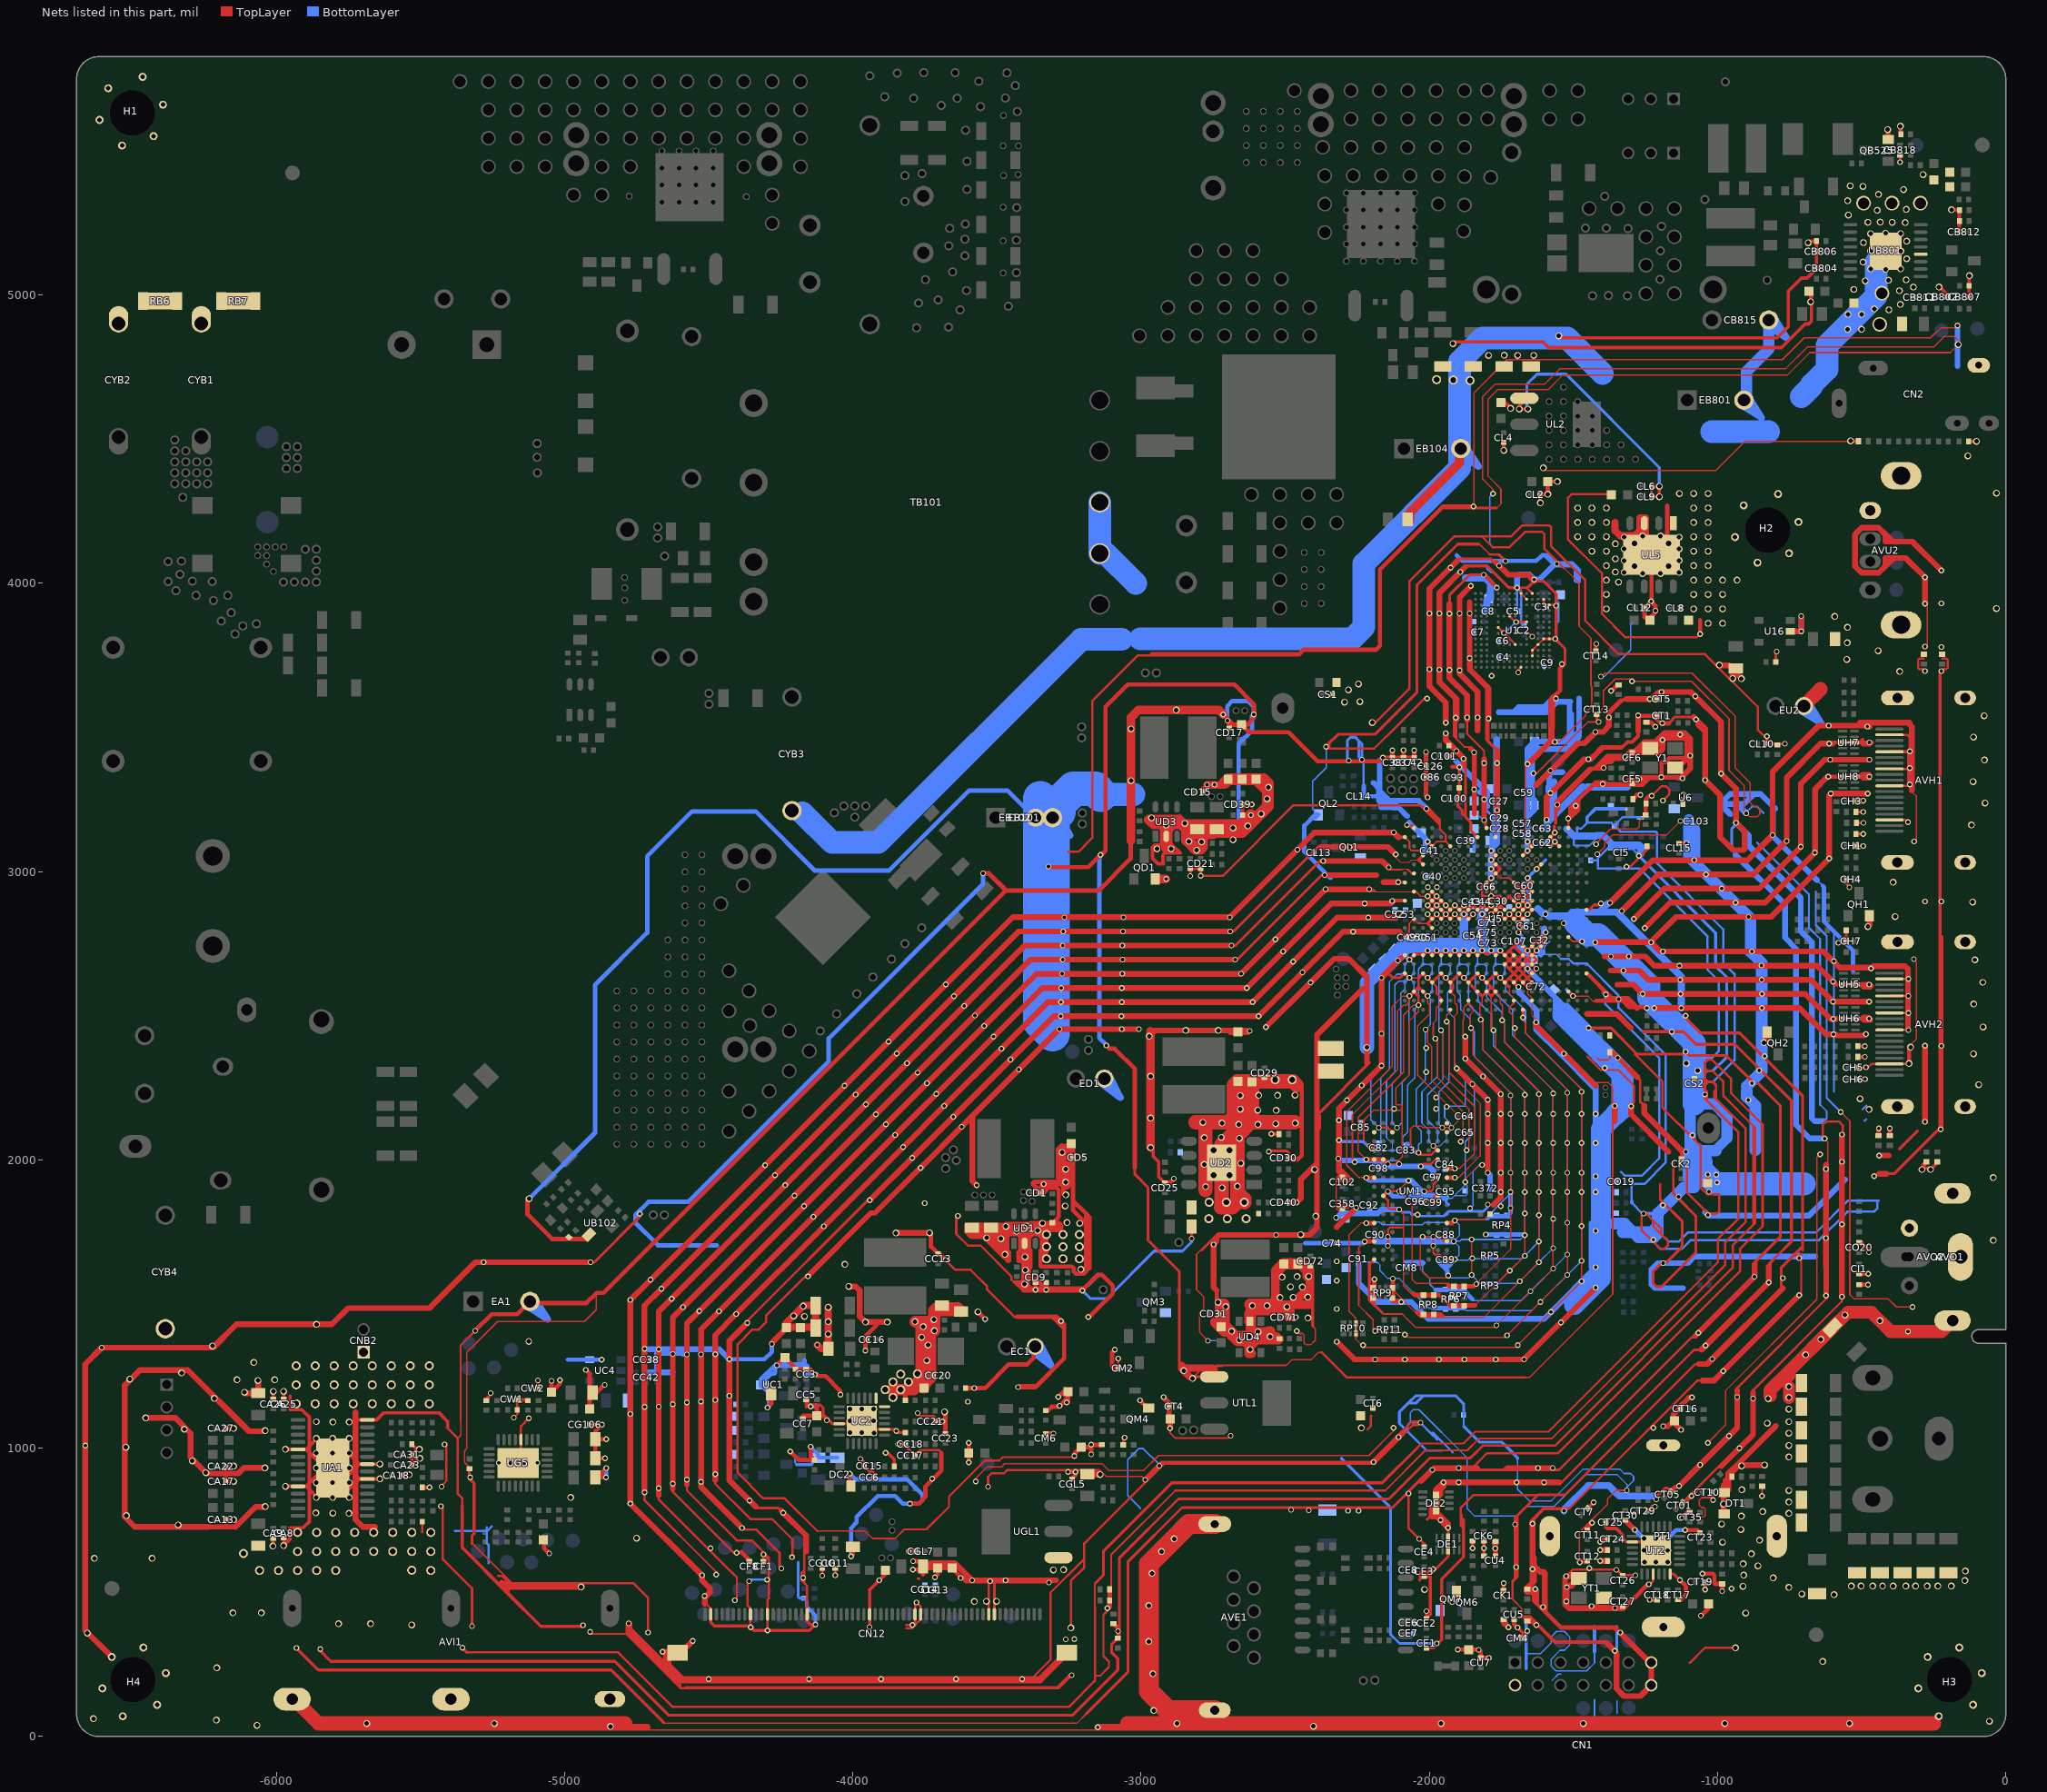
[diagram p0: the nets of this part, all layers, seen from the top]
# Altium PCB MISC84395.PcbDoc (part 13 of 26)
Units mil, origin at the board's own origin, x right, y up, seen from the top; angles counter-clockwise.
Board outline 6692.91 x 5826.77 mil, 2 copper layers (TopLayer, BottomLayer), stack 61.855 mil thick; 951 components, 565 nets, 4374 pads, 1804 vias.
Unrouted connection lines stored in the file: 1.

## Via types
v1: diameter 19.68, hole 11.81, TopLayer to BottomLayer, tented both sides, 1262 vias
v2: diameter 23.62, hole 15.75, TopLayer to BottomLayer, tented both sides, 524 vias
v3: diameter 31.5, hole 19.68, TopLayer to BottomLayer, tented both sides, 11 vias
v4: diameter 24, hole 16, TopLayer to BottomLayer, tented both sides, 6 vias
v5: diameter 19, hole 11.81, TopLayer to BottomLayer, tented both sides, 1 vias

## Nets (pads, with @x,y where several pads share a name; then routed paths per layer and width w, separated by ;. In a path a pad name is that pad's centre, name@x,y a point inside that pad or via, vN(x,y) a via of type N, cw(c..) or ccw(c..) an arc to the next point about the centre after c; other vN are vias at no path point) (continued)
GND: AVE1.9 AVE1.10 AVH1.2 AVH1.5 AVH1.8 AVH1.11 AVH1.17 AVH1.20 AVH1.21 AVH1.22 AVH1.23 AVH2.2 AVH2.5 AVH2.8 AVH2.11 AVH2.17 AVH2.20 AVH2.21 AVH2.22 AVH2.23 AVI1.2 AVI1.4 AVI1.6 AVO1.2 AVO2.3 AVO2.4 AVO2.5 AVU2.4 AVU2.5 AVU2.6 C1.1 C2.1 C3.1 C4.1 C5.1 C6.1 C7.1 C8.1 C9.2 C25.1 C26.1 C27.1 C28.1 C29.1 C30.1 C31.1 C32.1 C33.1 C34.1 C35.1 C36.1 C37.1 C38.1 C39.1 C40.1 C41.1 C42.1 C43.1 C44.1 C45.1 C46.1 C47.1 C48.1 C49.1 C50.1 C51.1 C52.1 C53.1 C54.2 C55.1 C56.1 C57.1 C58.1 C59.1 C60.1 C61.1 C62.1 C63.1 C64.2 C65.1 C66.2 C71.1 C72.1 C73.1 C74.1 C75.1 C80.1 C81.1 C82.1 C83.1 C84.1 C85.1 C86.2 C87.1 C88.1 C89.1 C90.1 C91.1 C92.1 C93.1 C94.1 C95.1 C96.1 C97.1 C98.1 C99.1 C100.1 C101.2 C102.2 C103.1 C104.1 C105.1 C106.1 C107.1 C108.1 C126.2 C358.1 C372.1 CA1.1 CA2.1 CA8.1 CA9.1 CA13.1 CA17.2 CA18.2 CA22.1 CA23.2 CA25.2 CA26.1 CA27.2 CA31.2 CB802.1 CB803.1 CB804.1 CB805.1 CB806.1 CB807.2 CB811.2 CB812.1 CB813.1 CB814.2 CB815.2 CB816.2 CB818.1 CB819.2 CC1.1 CC2.1 CC3.2 CC4.2 CC5.2 CC6.1 CC7.1 CC8.2 CC9.2 CC10.2 CC11.2 CC12.2 CC13.1 CC14.1 CC15.1 CC16.1 CC17.1 CC18.1 CC19.2 CC20.1 CC21.2 CC22.2 CC23.1 CC28.2 CC29.2 CC30.2 CC33.1 CC34.1 CC36.2 CC38.2 CC42.2 CC43.1 CD1.1 CD2.1 CD4.2 CD5.2 CD6.2 CD8.1 CD9.2 CD13.2 CD14.2 CD15.2 CD17.2 CD18.2 CD19.2 CD20.2 CD21.2 CD23.1 CD24.1 CD25.1 CD26.1 CD28.1 CD29.2 CD30.2 CD31.1 CD39.2 CD40.2 CD45.2 CD69.1 CD71.1 CD72.1 CD73.2 CD74.2 CE1.1 CE2.1 CE3.1 CE4.1 CE5.2 CE6.1 CE7.1 CE8.2 CF1.1 CF5.2 CF6.2 CF8.1 CG1.2 CG2.2 CG3.2 CG10.1 CG11.1 CG12.1 CG13.1 CG14.1 CG103.1 CG104.2 CG105.1 CG106.1 CGL4.1 CGL5.2 CGL6.2 CGL7.2 CGL49.2 CH1.2 CH3.1 CH4.1 CH5.2 CH6.1 CH7.1 CI1.1 CI5.1 CK1.2 CK2.2 CK6.1 CL1.1 CL2.2 CL3.2 CL4.2 CL5.1 CL6.1 CL7.1 CL8.1 CL9.1 CL10.1 CL11.2 CL12.2 CL13.1 CL14.1 CL15.1 CM2.2 CM3.1 CM4.1 CM6.1 CM7.1 CM8.1 CM9.1 CN1.2 CN1.13 CN1.14 CN2.1 CN12.2 CN12.9 CN12.12 CN12.19 CN12.30 CN12.38 CN12.39 CN12.51 CN12.52 CN12.61 CN12.62 CNB2.1 CO19.1 CO20.1 CS1.2 CS2.2 CT01.1 CT1.2 CT3.1 CT4.2 CT05.1 CT5.1 CT6.1 CT7.1 CT8.2 CT10.1 CT11.1 CT12.1 CT13.1 CT14.2 CT15.1 CT16.1 CT17.1 CT18.2 CT19.2 CT23.2 CT24.2 CT25.1 CT26.1 CT27.1 CT29.1 CT30.1 CT35.2 CT41.1 CT42.1 CT43.1 CT44.1 CT45.1 CT46.1 CT47.1 CT48.1 CT49.1 CT50.1 CT55.1 CT67.1 CT68.1 CT70.1 CU1.1 CU4.1 CU5.1 CU6.2 CU7.2 CU.2 CW1.1 CW2.2 CYB1.2 CYB2.2 CYB3.2 CYB4.2 D4.A D5.A D11.A D12.A D13.A D14.A DA1.A DA2.A DC2.3 DE1.GND DE2.EPAD@-1977,809.63 DH1.A DH2.A DH3.A DH4.A DH5.A DH6.A DI1.A DI2.A DI04.A DI4.A DK1.A DK3.A DO1.A DO7.A DT1.1 DT1.3 DT2.A DT3.A DT4.A DU1.A DU2.A DU3.A DU4.A DU5.A DU6.A DU7.A DU8.A DU9.A DV1.A DV2.A DV3.A DV4.A EA1.2 EB101.2 EB102.2 EB104.2 EB801.2 EC1.2 ED1.2 EU2.2 GND_JP1.JP_2K GND_JP2.JP_2K H1.1 H1.2 H1.3 H1.4 H1.5 H1.6 H2.1 H2.2 H2.3 H2.4 H2.5 H2.6 H3.1 H3.2 H3.3 H3.4 H3.5 H3.6 H4.1 H4.2 H4.3 H4.4 H4.5 H4.6 L3.2 LT2.2 LT5.1 MR313.1 P1.1 P1.2 pad.VIA5@-296.76,5318.37 pad.VIA5@-321,5027 pad.VIA5@-344.19,5125.37 pad.VIA5@-344.19,5186.37 pad.VIA5@-345.69,5296.87 pad.VIA5@-346.19,5052.37 pad.VIA5@-349.69,5250.87 pad.VIA5@-355,5365 pad.VIA5@-366.19,4967.37 pad.VIA5@-369.19,5014.37 pad.VIA5@-394.69,5251.79 pad.VIA5@-395.19,5318.37 pad.VIA5@-406,4948 pad.VIA5@-407.19,5050.87 pad.VIA5@-430.19,5005.87 pad.VIA5@-436.19,5252.37 pad.VIA5@-438,4898 pad.VIA5@-442,5349 pad.VIA5@-446.19,5293.37 pad.VIA5@-457,4952 pad.VIA5@-479.19,5251.87 pad.VIA5@-488.19,5048.37 pad.VIA5@-493.61,5318.37 pad.VIA5@-494.19,5181.37 pad.VIA5@-495.19,5113.87 pad.VIA5@-496,5376 pad.VIA5@-501,4881 pad.VIA5@-501,4933 pad.VIA5@-528,5019 pad.VIA5@-540,5378 pad.VIA5@-546.69,5276.87 pad.VIA5@-548,4933 pad.VIA5@-549,4881 pad.VIA5@-549.19,5326.87 pad.VIA5@-933.04,4011 pad.VIA5@-983.04,3861 pad.VIA5@-983.04,3911 pad.VIA5@-983.04,3961 pad.VIA5@-983.04,4011 pad.VIA5@-1033.04,3861 pad.VIA5@-1033.04,3911 pad.VIA5@-1033.04,3961 pad.VIA5@-1033.04,4011 pad.VIA5@-1033.04,4061 pad.VIA5@-1033.04,4111 pad.VIA5@-1033.04,4161 pad.VIA5@-1033.04,4211 pad.VIA5@-1033.04,4261 pad.VIA5@-1033.04,4311 pad.VIA5@-1083.04,3911 pad.VIA5@-1083.04,3961 pad.VIA5@-1083.04,4011 pad.VIA5@-1083.04,4061 pad.VIA5@-1083.04,4111 pad.VIA5@-1083.04,4161 pad.VIA5@-1083.04,4211 pad.VIA5@-1083.04,4261 pad.VIA5@-1083.04,4311 pad.VIA5@-1133.04,4311 pad.VIA5@-1344,4004 pad.VIA5@-1355,4039 pad.VIA5@-1355,4084.5 pad.VIA5@-1355,4137 pad.VIA5@-1386,3911 pad.VIA5@-1386,3961 pad.VIA5@-1386,4011 pad.VIA5@-1386,4061 pad.VIA5@-1386,4111 pad.VIA5@-1386,4161 pad.VIA5@-1386,4211 pad.VIA5@-1386,4261 pad.VIA5@-1436,4111 pad.VIA5@-1436,4161 pad.VIA5@-1436,4211 pad.VIA5@-1436,4261 pad.VIA5@-1486,4161 pad.VIA5@-1486,4211 pad.VIA5@-1486,4261 pad.VIA5@-1638,4790 pad.VIA5@-1694,4790 pad.VIA5@-1740,4791 pad.VIA5@-1795,4790 pad.VIA5@-1859,4703 pad.VIA5@-1917,4705 pad.VIA5@-1975,4706 pad.VIA5@-2476,2278 pad.VIA5@-2535,2278 pad.VIA5@-2636,1796 pad.VIA5@-2642,1853 pad.VIA5@-2681,3110 pad.VIA5@-2701,1796 pad.VIA5@-2704,1853 pad.VIA5@-2764,1853 pad.VIA5@-2765,1796 pad.VIA5@-2790,3103 pad.VIA5@-2807,3074 pad.VIA5@-2834,3105 pad.VIA5@-2848,3166.69 pad.VIA5@-2895.85,3078.43 pad.VIA5@-2913,3161 pad.VIA5@-2944.83,3078.43 pad.VIA5@-2964,3186 pad.VIA5@-3214,1657 pad.VIA5@-3214,1699 pad.VIA5@-3214,1741 pad.VIA5@-3271,1657 pad.VIA5@-3271,1699 pad.VIA5@-3271,1741 pad.VIA5@-3328,1657 pad.VIA5@-3328,1699 pad.VIA5@-3328,1741 pad.VIA5@-3776,1258 pad.VIA5@-3807,1230 pad.VIA5@-3833.87,1203.13 pad.VIA5@-3833.87,1256.87 pad.VIA5@-3860.74,1176.26 pad.VIA5@-3860.74,1230 pad.VIA5@-3887.61,1203.13 pad.VIA5@-5463.94,576 pad.VIA5@-5463.94,642 pad.VIA5@-5463.94,708 pad.VIA5@-5468.95,1154 pad.VIA5@-5468.95,1220 pad.VIA5@-5468.95,1286 pad.VIA5@-5529.94,642 pad.VIA5@-5529.94,708 pad.VIA5@-5530,577 pad.VIA5@-5534.95,1154 pad.VIA5@-5534.95,1220 pad.VIA5@-5534.95,1286 pad.VIA5@-5595.94,642 pad.VIA5@-5595.94,708 pad.VIA5@-5600.95,1154 pad.VIA5@-5600.95,1220 pad.VIA5@-5600.95,1286 pad.VIA5@-5661.94,642 pad.VIA5@-5661.94,708 pad.VIA5@-5666.94,1154 pad.VIA5@-5666.94,1220 pad.VIA5@-5666.95,1286 pad.VIA5@-5727.94,642 pad.VIA5@-5727.94,708 pad.VIA5@-5732.94,1154 pad.VIA5@-5732.94,1220 pad.VIA5@-5732.94,1286 pad.VIA5@-5793.94,576 pad.VIA5@-5793.94,642 pad.VIA5@-5793.94,708 pad.VIA5@-5798.94,1154 pad.VIA5@-5798.94,1220 pad.VIA5@-5798.94,1286 pad.VIA5@-5859.94,576 pad.VIA5@-5859.94,642 pad.VIA5@-5859.94,708 pad.VIA5@-5864.94,1154 pad.VIA5@-5864.94,1220 pad.VIA5@-5864.94,1286 pad.VIA5@-5925.94,576 pad.VIA5@-5925.94,642 pad.VIA5@-5925.94,708 pad.VIA5@-5930.94,1154 pad.VIA5@-5930.94,1220 pad.VIA5@-5930.94,1286 pad.VIA5@-5991.94,576 pad.VIA5@-6057.94,576 pad.VIA5@-6113.94,635 PT1.1 PT1.2 PT1.3 PT1.4 QB525.E QD1.S QH1.E QH2.E QL1.E QL2.E QM3.E QM4.E QM6.E QM7.E R3.1 R11.1 R26.1 R28.1 R33.1 R37.1 R47.1 R49.2 R50.2 R52.1 RA19.1 RA21.1 RA31.1 RB6.1 RB6.2 RB6.3 RB7.1 RB7.2 RB7.3 RB134.1 RB140.2 RB803.1 RB812.1 RB818.2 RB819.2 RB820.2 RB821.2 RB822.1 RB827.1 RB834.1 RC3.1 RC7.2 RC12.1 RC17.1 RC18.1 RC24.1 RC26.1 RC27.1 RC31.1 RD4.1 RD9.1 RD16.1 RD27.2 RD28.2 RD51.1 RG2.1 RG3.1 RG4.1 RG7.2 RG8.2 RG9.2 RG30.2 RI5.1 RI9.2 RI12.2 RL8.1 RL10.2 RL11.2 RM3.2 RM9.2 RM11.1 RM14.2 RO4.1 RP3.5 RP3.6 RP4.1 RP4.2 RP4.7 RP4.8 RP5.3 RP5.4 RP6.1 RP6.2 RP6.7 RP6.8 RP7.1 RP7.2 RP7.7 RP7.8 RP8.1 RP8.2 RP8.7 RP8.8 RP9.1 RP9.2 RP9.7 RP9.8 RP10.3 RP10.4 RP11.5 RP11.6 RS1.1 RS2.2 RU10.1 RW2.1 TB101.8 TB101.9 U1.A6 U1.C4 U1.D4 U1.E3 U1.E7 U1.F1 U1.F2 U1.G5 U1.H10 U1.J5 U1.K8 U1.M1 U1.M2 U1.N2 U1.N5 U1.P4 U1.P6 U5.A8 U5.A16 U5.AA3 U5.AA12 U5.AA20 U5.B7 U5.B9 U5.B14 U5.B17 U5.C3 U5.C11 U5.C12 U5.C13 U5.C16 U5.C19 U5.C20 U5.D7 U5.D8 U5.D9 U5.D10 U5.D12 U5.D14 U5.D16 U5.D18 U5.E1 U5.E7 U5.E11 U5.E13 U5.E15 U5.E17 U5.E19 U5.E21 U5.F7 U5.F8 U5.F9 U5.F10 U5.G7 U5.G8 U5.G9 U5.G10 U5.G11 U5.G13 U5.G14 U5.G15 U5.G16 U5.G17 U5.G18 U5.G19 U5.G20 U5.G21 U5.H6 U5.H7 U5.H8 U5.J3 U5.J6 U5.J21 U5.K8 U5.K18 U5.L8 U5.L9 U5.L10 U5.L12 U5.L14 U5.L15 U5.L16 U5.L17 U5.L18 U5.L20 U5.M1 U5.M7 U5.M8 U5.M9 U5.M10 U5.M11 U5.M12 U5.M13 U5.M14 U5.M15 U5.M16 U5.M17 U5.M18 U5.N7 U5.N8 U5.N9 U5.N10 U5.N17 U5.N18 U5.N21 U5.P7 U5.P8 U5.P18 U5.P20 U5.R7 U5.R9 U5.R12 U5.R21 U5.T11 U5.T20 U5.U6 U5.U11 U5.U19 U5.V8 U5.V11 U5.V19 U5.W4 U5.W5 U5.W7 U5.W16 U5.W18 U5.Y5 U5.Y11 U5.Y13 U5.Y21 U6.1 U16.2 UA1.6 UA1.8 UA1.14 UA1.19 UA1.24 UA1.EPAD UB102.A UB801.4 UB801.17 UC1.3 UC2.4 UC2.14 UC2.18 UC2.19 UC2.25 UC4.5 UD1.2 UD2.9 UD3.2 UD4.2 UG5.4 UG5.EPAD UGL1.1 UH5.GND UH6.GND UH7.GND UH8.GND UL2.1 UL5.1 UL5.3 UL5.EPAD UM1.A9 UM1.B1 UM1.B3 UM1.B9 UM1.D1 UM1.D8 UM1.E1 UM1.E2 UM1.E8 UM1.F9 UM1.G1 UM1.G8 UM1.G9 UM1.J2 UM1.J8 UM1.M1 UM1.M9 UM1.P1 UM1.P9 UM1.T1 UM1.T9 UT2.14 UT2.21 UT2.24 UT2.25 UTL1.1 Y1.2 Y1.4 YT1.2 YT1.4 | length 337716.2
  TopLayer w3.94: v1@-2216.58,2939.92 -2215.26,2938.6 -2207.22,2930.57 -2195.87,2930.57 ; v1@-2206.34,2941.05 -2195.87,2930.57 ; -2137.21,2886.78 -2134.38,2889.6 v1@-2129.06,2894.93 ; v1@-2122.15,3054.24 -2100.84,3032.93 -2069.18,3032.93 -2061.31,3040.81 -2037.68,3040.81 ; -2097.22,3006.58 -2094.49,3009.31 -2077.05,3009.31 -2075.46,3007.72 -2061.31,2993.56 U5.T20@-2053.43,2993.56 ; -2081.98,2536.87 -2080.99,2536.87 -2069.18,2548.68 v1(-2069.18,2568.36) ; -2070.66,2522.6 -2070.66,2523.58 -2057.37,2536.87 v1(-2037.69,2536.87) ; U5.P20@-2053.43,2930.57 -2184.51,2930.57 ; U5.V19@-2023.9,3056.56 U5.V19@-2021.94,3056.56 ; v1(-2006.19,2568.36) -2006.19,2544.74 -2000.28,2538.84 -2000.28,2504.88 -2000.78,2504.39 ; -1977.16,2483.72 -1976.66,2484.21 -1976.66,2527.02 -1958.95,2544.74 U5.B17@-1958.94,2552.62 ; U5.C16@-1927.45,2584.12 -1911.7,2568.36 -1911.7,2544.74 -1903.83,2536.87 -1903.83,2507.83 -1904.32,2507.34 ; -1880.7,2486.67 -1880.21,2487.16 -1880.21,2528.99 -1864.46,2544.74 ; U5.B14@-1864.46,2552.62 -1864.46,2544.74 ; -1849.2,2513.25 -1848.71,2513.74 -1848.71,2528.99 -1864.46,2544.74 ; -1824.6,2506.85 -1825.09,2507.34 -1825.09,2536.87 -1817.21,2544.74 -1817.21,2568.36 ; U5.Y11@-1769.97,3119.55 -1769.97,3196.08 ; v1(-1747.82,2484.21) -1746.35,2485.69 -1746.35,2536.87 -1754.22,2544.74 -1754.22,2568.36 ; -1722.23,2512.75 -1722.73,2513.25 -1722.73,2528.99 -1706.98,2544.74 U5.B9@-1706.98,2552.62 ; -1667.47,3182.22 -1667.61,3182.08 -1667.61,3135.3 -1659.73,3127.42 v1(-1659.73,3103.8) ; U5.B7@-1643.98,2552.62 -1643.98,2500.95 -1641.52,2498.49 ; -2195.87,2930.57 -2189.65,2930.57 ; -2195.87,2930.57 -2195.87,2936.79 ; -2195.87,2936.79 -2189.65,2930.57 ; -2195.87,2936.79 -2195.87,2937.74 ; -2195.87,2937.74 -2195.65,2937.74 -2188.48,2930.57 ; -2195.87,2937.74 -2195.87,2941.93 -2184.51,2930.57 ; -2189.65,2930.57 -2188.48,2930.57 ; -2188.48,2930.57 -2184.51,2930.57 ; -1754.22,2568.36 U5.C11@-1769.97,2584.12 -1754.22,2568.36
  TopLayer w4: v1(-1404.77,2889.43) v1@-1399.93,2884.58
  TopLayer w4.92: C358.1@-2301.47,1823.95 -2316.23,1823.95 -2323.61,1831.34 -2323.61,1937.11 -2313.77,1946.95 C102.2@-2301.47,1946.95 ; v1(-2259.14,1992.58) -2267.02,2000.45 -2267.02,2156.95 -2109.54,2314.43 -2109.54,2517.18 -2089.85,2536.87 -2081.98,2536.87 ; RP10.4@-2254.71,1389.73 -2254.71,1376.93 -2227.64,1349.86 -1701.07,1349.86 v1(-1472.23,1578.7) -1472.23,2245.53 -1666.62,2439.92 -1666.62,2475.06 -1675.48,2483.92 v1(-1675.48,2493.56) ; RP10.3@-2254.71,1433.03 -2254.71,1450.75 -2279.32,1475.36 -2279.32,1738.64 -2237,1780.96 v1(-2218.79,1780.96) ; v1(-2224.69,1716.49) -2244.87,1696.31 -2244.87,1495.04 -2195.66,1445.83 -2195.66,1413.84 -2183.35,1401.54 -2092.31,1401.54 v1(-2084.93,1394.15) -2075.09,1384.31 -1737.99,1384.31 v1(-1730.6,1391.69) v1(-1614.95,1507.34) v1(-1521.44,1600.85) v1(-1521.45,2233.23) -1521.45,2243.08 -1703.53,2425.16 v1(-1703.53,2457.14) -1710.91,2464.52 -1710.91,2501.43 -1722.23,2512.75 ; v1(-2218.79,1938.44) -2243.89,1938.44 -2286.7,1981.26 -2286.7,2166.79 -2129.22,2324.27 -2129.22,2530.96 -2091.82,2568.36 v1(-2069.18,2568.36) ; v1(-2218.79,2001.43) -2247.33,2029.98 -2247.33,2147.1 -2089.85,2304.58 -2089.85,2501.43 -2070.66,2520.63 -2070.66,2522.6 ; v1(-2206.98,2048.68) -2227.65,2069.35 -2227.65,2137.26 -2193.2,2171.71 -2094.77,2171.71 ; -2162.65,1468.53 -2159.63,1465.51 -2094.77,1465.51 -2048.02,1418.76 -1774.88,1418.76 v1(-1767.51,1426.14) v1(-1649.4,1544.25) v1(-1570.66,1622.99) -1570.66,2240.61 -1740.44,2410.4 -1740.44,2476.84 v1(-1747.82,2484.21) ; v1(-2143.99,1985.69) -2118.4,1985.69 -2111.5,1992.58 -2094.77,2009.31 -2094.77,2171.71 ; RP9.1@-2126.76,1549.17 -2126.27,1548.68 -2030.79,1453.21 -1811.8,1453.21 v1(-1686.31,1578.7) v1(-1619.87,1645.14) -1619.87,2238.15 -1769.97,2388.25 -1769.97,2442.38 -1784.73,2457.14 -1784.73,2518.66 -1785.72,2519.64 -1785.72,2568.36 ; v1(-2104.62,1828.21) -2089.85,1813.44 -2089.85,1765.21 ; -2096.74,1765.21 -2089.85,1765.21 ; v1(-2072.63,1928.11) -2104.62,1896.12 v1(-2104.62,1891.2) -2060.32,1846.91 -2060.32,1586.09 -2045.56,1571.32 -1934.83,1571.32 -1924.99,1561.48 ; v1(-2037.69,2025.06) -2065.25,2052.62 -2065.25,2107.73 -2055.4,2117.58 -2027.84,2117.58 -2021.94,2111.67 v1(-1955.01,2111.67) ; v1(-2037.69,2536.87) -2037.69,2514.23 -2070.17,2481.75 -2070.17,2294.74 -2116.92,2248 -2116.92,2191.39 -2094.77,2191.39 -2094.77,2171.71 ; v1(-2013.57,2452.22) -2006.19,2444.84 -2006.19,2407.93 -1991.43,2393.17 -1991.43,2275.06 -1883.16,2166.79 -1883.16,2071.32 v1(-1891.03,2063.44) ; -2000.78,2504.39 -2040.64,2464.52 -2040.64,2294.74 -1969.28,2223.39 -1934.82,2188.94 -1902.84,2156.95 -1902.84,2132.34 v1(-1923.51,2111.67) ; v1(-1986.51,1733.72) v1(-2023.41,1733.72) -2030.8,1726.34 -2030.8,1620.54 -2001.27,1591.01 -1942.21,1591.01 v1(-1934.83,1598.38) ; -1977.16,2483.72 -1986.51,2474.37 -1986.51,2427.62 v1(-1979.12,2420.23) -1971.74,2412.86 -1971.74,2284.9 -1863.47,2176.64 -1863.47,2041.3 ; v1(-1959.44,2449.76) -1952.06,2442.38 -1952.06,2294.74 -1843.79,2186.47 -1843.79,2022.11 -1895.95,1969.94 v1(-1911.7,1969.94) ; U5.A16@-1927.45,2521.12 -1927.45,2513.74 -1939.75,2501.43 v1(-1939.75,2479.29) -1932.37,2471.91 -1932.37,2304.58 -1824.1,2196.32 -1824.1,2013.74 -1899.4,1938.44 v1(-1911.7,1938.44) ; -1924.99,1495.04 -1966.82,1536.87 -2062.78,1536.87 -2089.85,1563.93 -2089.85,1765.21 ; v1(-1911.7,1789.82) -1908.75,1792.77 -1809.03,1792.77 MR313.1@-1789.34,1812.46 ; v1(-1905.3,2316.89) -1912.69,2316.89 -1912.69,2498.97 -1904.32,2507.34 ; -1880.7,2486.67 -1883.16,2484.21 -1883.16,2427.62 v1(-1875.78,2427.62) ; v1(-1875.77,1923.19) -1875.77,1933.82 -1872.68,1936.91 -1827.35,1982.24 v1(-1816.72,1982.24) ; v1(-1853.63,1600.85) v1(-1853.63,1723.88) ; -1849.2,2513.25 -1858.55,2503.89 -1858.55,2459.6 -1848.71,2449.76 -1848.71,2363.64 -1718.3,2233.23 -1718.3,1689.43 -1846.24,1561.48 ; -1841.33,1495.04 v1(-1720.76,1615.61) v1(-1669.08,1667.28) -1669.08,2235.69 -1814.26,2380.86 -1814.26,2479.29 v1(-1821.64,2486.67) -1821.64,2503.89 -1824.6,2506.85 ; -1659.73,2599.86 -1659.73,2576.24 -1643.98,2560.49 U5.B7@-1643.98,2552.62 ; -1641.52,2498.49 -1629.71,2486.67 v1(-1629.71,2476.83) ; v1(-1955.01,2111.67) v1(-1923.51,2111.67) ; v1(-1955.01,2111.67) UM1.B9@-1939.26,2095.93 v1(-1923.51,2111.67) ; v1(-1955.01,2111.67) UM1.A9@-1939.26,2127.42 v1(-1923.51,2111.67)
  TopLayer w5: RG3.1@-5330,929.27 -5330,933.42 -5347.34,950.77 -5347.34,990.66 -5339,999 -5339,1332.53 -5232.03,1439.5 -4930.57,1439.5 -4889.84,1480.23 -4889.84,1532 ; -5321.04,669.04 -5319.04,669.04 -5183.5,533.5 -5170.5,533.5 ; -5225,532.5 -5220,537.5 -5192.5,537.5 -5188.5,533.5 ; -5197,539.5 -5191,533.5 -5170.5,533.5 ; -4714,32.5 -4704.5,23 -3112,23 ; v1(-4710,361) -4710,483 -4760.5,533.5 -5170.5,533.5 ; -4655.5,48.5 -4653,46 -3223.79,46 -3190,79.79 ; -4123.13,713.09 -3958.28,713.09 -3932.19,687 -3853,687 -3836,704 ; v1@-3574.71,884.84 -3574.71,894.52 -3534.62,934.61 -3484.7,934.61 -3473.3,946 -3135.14,946 -3111.14,922 -2992.34,922 -2939.34,975 -2209.41,975 -2124.13,1060.27 v1(-2124.13,1070.66) ; CGL4.1@-3209,926 -3145,926 -3121,902 -2997.45,902 v1(-2985.45,890) ; v2@-2817.5,1247.55 -2782.21,1282.84 -2717.59,1282.84 -2712.94,1287.5 -2705.5,1287.5 ; -2778.29,1383 v1(-2768.12,1372.82) -2797.5,1402.21 -2797.5,1470.55 -2782.66,1485.39 -2782.66,1524.61 -2807.5,1549.45 -2807.5,1672.62 -2794.06,1686.06 ; UTL1.1@-2746.27,1247.55 -2746.27,1271.73 -2746.27,1281.73 -2740.5,1287.5 -2705.5,1287.5 ; v1(-2460,1406) v1@-2460,1403 ; v1@-2457,1400 v1@-2460,1403 ; -2445.6,1397.6 -2439.3,1397.6 ; -2443.21,1397.6 -2439.3,1397.6 ; -2405,1424 -2395.5,1414.5 -2395.5,1374.76 -2411.76,1358.5 -2428,1358.5 -2434.91,1365.41 -2434.91,1393.21 -2439.3,1397.6 ; -2382.57,2106.37 -2380.07,2108.87 ; -2374.28,1332.89 -2384.01,1332.89 -2410.41,1306.5 -2477.5,1306.5 -2496.5,1287.5 -2705.5,1287.5 ; UM1.B1@-2191.23,2095.93 v1(-2175.48,2111.67) ; -2078.45,3007.72 -2075.46,3007.72 -2073.96,3006.22 ; -2070.34,2798.55 -2070.34,2819.17 -2069.84,2819.67 U5.L20@-2053.43,2836.08 ; v1(-2069.18,2631.36) -2037.69,2631.36 ; -2045.56,2930.57 -2029.81,2914.82 v1(-2006.19,2914.82) ; -2029.81,2820.34 -2006.19,2820.34 ; v1@-1846,4266.84 -1846,4659.14 -1730.02,4775.12 -775.59,4775.12 -699.71,4851 -261.43,4851 -226.43,4886 -176,4886 v1(-168,4894) ; -1829.83,4136 -1826.3,4136 -1789.45,4099.16 ; v1(-1817.21,2725.84) -1817.21,2820.34 U5.L12@-1801.46,2836.08 ; v1(-1779,4311) -1779,4325.86 -1816,4362.86 -1816,4646.72 -1771.72,4691 -1599.86,4691 ; U5.T11@-1769.97,2993.56 -1754.22,2977.82 -1722.72,2977.82 U5.R9@-1706.98,2962.07 ; -1769.97,3196.08 -1764.97,3201.08 ; -1766,4261 -1751.66,4275.34 -1751.66,4326.8 -1796,4371.14 -1796,4638.43 -1763.43,4671 -1588.61,4671 -1537.11,4722.5 -757.5,4722.5 -680,4800 -193,4800 v2(-165,4828) ; -1722.72,2599.86 -1722.72,2576.24 -1706.98,2560.49 U5.B9@-1706.98,2552.62 ; -1697.31,567.46 -1697.31,552.5 -1697.31,549 -1710.33,535.98 ; -1667.47,3182.22 -1667.47,3363.08 ; -1667,1245.11 -1653.37,1245.11 -1364.17,1534.3 -1364.17,2127.33 ; DU6.A@-1660,403.27 -1670.94,414.2 -1678.33,421.59 -1678.33,442.67 -1710.33,474.67 ; v1(-1638.71,3340.34) -1628.32,3340.34 -1449.93,3518.74 v1(-1412.65,3518.74) ; v2(-1605,4400) -1595.5,4390.5 -1007.15,4390.5 -905.65,4492 -549.77,4492 -544.07,4486.3 v2@-537.69,4492.69 ; -1599.33,4119.95 -1480.65,4001.27 -1480.65,3850.63 -1439.71,3809.69 -1439.71,3644.38 -1436.34,3641.02 ; -1590.14,4700.72 -1599.86,4691 ; v1(-1564.65,3449.74) -1549.12,3449.74 -1458.43,3540.43 -1458.43,3551.1 -1436.99,3572.53 -1436.99,3640.37 -1436.34,3641.02 ; v1@-1534.41,2821 v1(-1533.99,2820.58) ; U5.C3@-1518,2584.12 -1502.57,2568.68 v1(-1502.25,2568.68) ; v1@-1500.77,2567.21 -1448.97,2567.21 -1431.5,2549.74 -1369.75,2549.74 ; v1@-1479.47,602.53 -1479.47,707.96 -1454.27,733.16 -1382.66,804.77 -1382.66,823.34 -1352,854 v1(-1315,854) ; -1465.51,2301.33 -1456.12,2301.33 -1451.2,2296.4 ; -1436.34,3591.09 -1436.34,3641.02 ; -1426.83,2269 -1380.32,2269 -1364.5,2253.19 -1364.5,2173.17 ; v1@-1422.98,3096.01 v1@-1421.69,3097.31 ; v1(-1421.69,3094.72) v1@-1421.69,3097.31 ; CT13.1@-1419.65,3545.01 -1419.65,3545.35 -1396,3569 -1396,3627 -1355.48,3667.52 -1304.33,3667.52 v1(-1296.99,3660.18) -1090.41,3660.18 -960.65,3530.41 -960.65,3351.27 -908.49,3299.12 -908.49,3203.66 -906.83,3202 v1(-900.83,3202) -888.49,3189.66 -863.65,3189.66 -853.49,3199.82 -853.49,3214.18 -863.65,3224.34 -873.33,3224.34 -887.49,3238.51 -887.49,3307.82 -939.65,3359.97 -939.65,3539.11 -1089.06,3688.52 -1390.48,3688.52 -1403,3676 v1(-1405,3676) ; -1418.7,2354.41 -1410.63,2346.34 -1380.49,2346.34 -1373.79,2353.05 DU1.A@-1373.79,2372.74 ; v1(-1418,3060) -1410.62,3067.38 -1410.36,3067.38 -1394.35,3083.4 -1394.35,3083.65 -1391.65,3086.35 -1391.65,3099.06 -1362.87,3127.84 -1176.16,3127.84 v1(-1129,3175) ; v1(-1369.67,3626.83) -1367.8,3626.83 -1363.9,3626.83 D13.A@-1343,3647.73 ; R3.1@-1249.77,3196.47 -1272.43,3173.82 -1272.43,3155.57 -1280.16,3147.84 -1371.15,3147.84 v1@-1421.69,3097.31 ; CT35.2@-1097,777.74 -1094.71,777.74 -1078.34,761.37 -1048.05,761.37 -1043.66,765.77 -1043.66,789.7 -1048.05,794.09 -1056.09,794.09 -1063.45,801.45 -1063.45,819.62 -1054.29,828.78 -1024.78,828.78 ; v1(-1034,1019) -973,1080 -973,1198.86 -655.5,1516.36 -655.5,2008.5 v1(-645,2019) ; CL10.1@-829.11,3435.3 CL10.1@-829.11,3443 ; v1(-629,2074.13) -617.66,2062.79 -617.66,1989.07 -624,1982.73 ; v1(-573.12,2166.27) -541.5,2134.65 -541.5,1532.5 -526.64,1517.64 -407.91,1517.64 -380.26,1490 v1(-324,1490) ; v1(-333.38,3301.79) -333.38,3284.38 -311.03,3262.03 -311.03,3111.56 v1(-318.59,3104) ; v2(-331,2391) -331,2398.52 -310.03,2419.49 -310.03,2685.03 -318,2693 v1@-318,2695 ; v1@-284,2897 v1@-281,2894 ; v1(-280.83,3780) -273.33,3787.5 -273.33,3921.5 v1(-280.83,3929) ; v2@-158.69,4834.69 -180,4856 -214,4856 -250,4820 -688.28,4820 -763.79,4744.5 -1546.36,4744.5 -1599.86,4691 ; -2794.06,1686.06 -2787.94,1686.06 -2743.13,1730.87 -2738.65,1730.87 -2749.25,1730.87 -2794.06,1686.06 ; v1@-2460,1403 -2454.6,1397.6 -2439.3,1397.6 ; -1710.33,474.67 -1712.67,477.02 -1712.67,537.15 -1710.33,539.49 -1710.33,535.98 ; -1710.33,474.67 -1710.33,535.98
  TopLayer w6: -5370.97,1034.8 -5359.5,1046.27 -5359.5,1110 ; -3449.84,1595.85 -3448.84,1594.85 -3448.84,1582.86 -3431.68,1565.7 ; v1@-2898.81,1070.19 -2898.81,1051.81 -2882.5,1035.5 -2697,1035.5 v1(-2689.5,1043) ; v1@-2138.56,3006.58 -2097.22,3006.58 ; U5.J21@-2084.93,2773.09 -2069.84,2788.18 -2069.84,2819.67 ; U5.L20@-2053.43,2836.08 -2037.68,2820.34 -2029.81,2820.34 ; v1@-1915.55,3539.74 -1915.55,3469.44 -1910.65,3464.54 ; -1910.65,3522.05 -1910.65,3464.54 ; v1@-1905.55,3527.15 -1905.55,3459.44 ; -1837.97,3233 -1837.97,3406.41 -1843.97,3412.41 v1(-1844.82,3413.26) -1844.82,3414.46 -1844.82,3422.94 -1854.63,3432.75 -1878.86,3432.75 -1905.55,3459.44 ; DU6.A@-1660,397.66 DU6.A@-1660,401.27 DU6.A@-1660,403.27 ; U1.E3@-1623.28,3787.34 U1.F2@-1603.6,3807.03 ; -1598,438.71 -1541.69,382.39 ; -1569.1,401.8 -1549.69,382.39 -1541.69,382.39 ; -1536.5,456.4 -1518.6,438.5 -1325.02,438.5 -1311,452.52 -1311,454.64 ; U5.J3@-1518,2773.09 -1502.27,2757.37 v1(-1470.58,2757.37) ; v1(-1338.43,360.58) -1351.25,373.39 ; -1329.56,442 -1323.64,442 -1314.37,451.27 ; CT27.1@-1329.29,451.27 -1318.61,451.27 -1314.37,451.27 ; -1310.84,465.36 -1311,465.2 -1311,458.88 -1311,454.64 ; -1294.36,481.84 -1248.14,528.06 v1(-1238.47,528.06) ; -1910.65,3464.54 -1905.55,3459.44 ; -1541.69,382.39 -1538.69,379.39 ; -1541.69,382.39 -1360.25,382.39 -1357.25,379.39 ; -1538.69,379.39 -1357.25,379.39 ; -1538.69,379.39 -1535.69,376.39 -1532.69,373.39 -1351.25,373.39 ; -1357.25,379.39 -1351.25,373.39 ; -1314.37,451.27 -1311,454.64
  TopLayer w7: -5360,1094.24 -5360,1357.5 v1(-5310,1407.5) ; v1(-4911,363) -4911,360.5 -4907,356.5 -4786.72,356.5 -4597.22,167 -3285.68,167 -3241,211.68 v1(-3241,213) ; -4416.41,566 -4402.34,551.93 -4402.34,479.66 v1(-4409,473) ; -3836,704 -3821.5,718.5 -3744.94,718.5 -3666.5,796.94 -3666.5,832.42 -3541.92,957 -3492,957 -3479.84,969.16 v1@-3231.43,969.16 ; v1(-3775,1122) -3764.66,1111.66 -3718,1111.66 -3714.26,1107.92 CC21.2@-3714.26,1093 ; -3159.95,211.5 -3141.02,211.5 -3111.46,241.06 -3111.46,260.16 -3130.33,279.02 -3130.33,422.11 -3103.5,448.94 -3103.5,631.23 -2881.23,853.5 -2152.69,853.5 -2013.69,992.5 -1868.56,992.5 -1827.72,1033.34 -1576.05,1033.34 -973.5,1635.89 -973.5,1636.6 ; -3159.95,449.81 -3159.95,450.52 -3160.45,451.02 -3160.45,531.87 -3152.91,539.41 ; U5.Y21@-2084.93,3119.55 -2069.34,3103.96 -2069.34,3081.44 -2060.37,3072.47 -2037.85,3072.47 U5.V19@-2021.94,3056.56 ; -2043.04,1000.62 -2027.16,1016.5 -1881.33,1016.5 -1840.49,1057.34 -1587.4,1057.34 -999.5,1645.25 -999.5,1647.37 ; U5.W18@-1990.44,3088.05 -1974.53,3103.96 -1943.36,3103.96 -1943.2,3104.12 ; -1943.2,3126.55 -1943.2,3104.12 ; U5.W16@-1927.45,3088.05 -1927.45,3088.38 -1943.2,3104.12 ; -1869.05,3522.91 -1869.05,3477.58 -1809.97,3418.5 -1809.97,3389.84 ; -1817.21,2886.04 -1817.21,2946.32 ; -1816.51,2914.99 -1786.04,2914.99 v1(-1785.72,2915.3) ; U5.R12@-1801.46,2962.07 -1785.72,2946.32 v1(-1785.72,2915.3) ; v1(-1785.72,2883.33) v1(-1785.72,2915.3) ; -1754.38,2914.99 -1785.4,2914.99 v1(-1785.72,2915.3) ; U1.K8@-1721.71,3885.77 -1701.78,3865.84 v1(-1699.21,3865.84) ; -1682.21,3984.34 -1682.34,3984.21 U1.P6@-1682.34,3964.51 U1.N5@-1662.65,3944.82 ; U1.G5@-1662.65,3826.71 -1655.08,3826.71 -1643.66,3815.29 v1(-1642.97,3815.29) ; -1452.63,2358.64 -1405.99,2312 -1384.83,2312 ; v1(-1391.83,2319) -1384.83,2312 ; v1@-1300.33,2188.41 -1290.49,2198.25 -1290.49,2258.11 -1344.38,2312 -1384.83,2312 ; v1(-846,834) DT4.A@-846,868.27 ; v1@-712,1658.36 -710.5,1656.86 v1@-710.5,1537.3